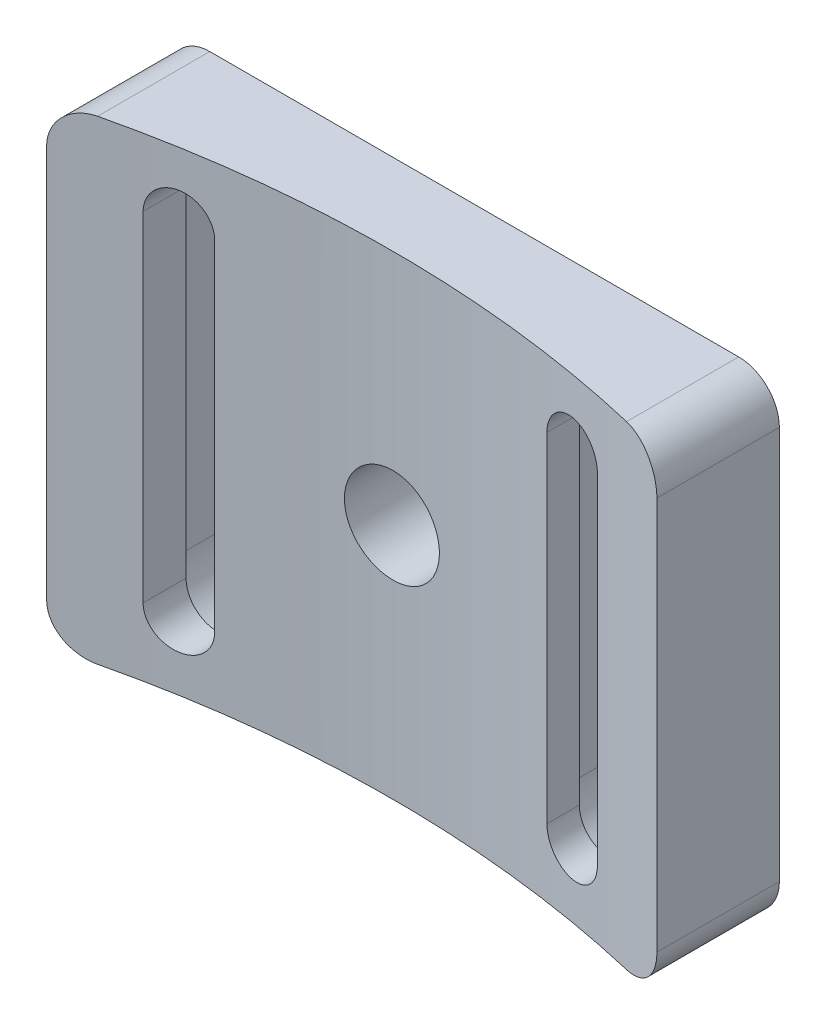
from build123d import *

# Parameters (mm, degrees)
BOSS_EXTRUDE1_DEPTH   = 35
FILLET1_R             = 3
M8X1_0_TAPPED_HOLE1_D = 7
CUT_EXTRUDE1_DEPTH    = 43.577310513
CUT_EXTRUDE2_DEPTH    = 4.5


with BuildPart() as part:
    # Sketch1 → Boss-Extrude1 (new body)
    with BuildSketch(Plane(origin=(0, 0, 0), x_dir=(1, 0, 0), z_dir=(0, 1, 0))):
        with BuildLine():
            Line((-22.5, 81.967981554), (-22.5, 91))
            Line((-22.5, 91), (22.5, 91))
            Line((22.5, 91), (22.5, 81.967981554))
            ThreePointArc((22.5, 81.967981554), (0, 85), (-22.5, 81.967981554))
        make_face()
    extrude(amount=BOSS_EXTRUDE1_DEPTH)

    # Fillet1
    fillet1_edges = [part.edges().sort_by_distance(p)[0] for p in [
        (22.5, 35, -86.483990777),
        (22.5, 0, -86.483990777),
        (-22.5, 0, -86.483990777),
        (-22.5, 35, -86.483990777),
    ]]
    fillet(fillet1_edges, radius=FILLET1_R)

    # M8x1.0 Tapped Hole1 (through all)
    with Locations(Plane(origin=(0, 0, -91), x_dir=(-1, 0, 0), z_dir=(0, 0, -1))):
        with Locations((0, 17.5)):
            Hole(M8X1_0_TAPPED_HOLE1_D / 2)

    # Sketch4 → Cut-Extrude1 (cut, through all)
    with BuildSketch(Plane(origin=(0, 0, -91), x_dir=(-1, 0, 0), z_dir=(0, 0, -1))):
        with BuildLine():
            Line((-12.25, 30), (-12.25, 5))
            ThreePointArc((-12.25, 5), (-14.5, 2.75), (-16.75, 5))
            Line((-16.75, 5), (-16.75, 30))
            ThreePointArc((-16.75, 30), (-14.5, 32.25), (-12.25, 30))
        make_face()
        with BuildLine():
            Line((16.75, 30), (16.75, 5))
            ThreePointArc((16.75, 5), (14.5, 2.75), (12.25, 5))
            Line((12.25, 5), (12.25, 30))
            ThreePointArc((12.25, 30), (14.5, 32.25), (16.75, 30))
        make_face()
    extrude(amount=-CUT_EXTRUDE1_DEPTH, mode=Mode.SUBTRACT)

    # Sketch5 → Cut-Extrude2 (cut)
    with BuildSketch(Plane(origin=(0, 0, -91), x_dir=(-1, 0, 0), z_dir=(0, 0, -1))):
        with BuildLine():
            Line((-10.5, 30), (-10.5, 5))
            ThreePointArc((-10.5, 5), (-14.5, 1), (-18.5, 5))
            Line((-18.5, 5), (-18.5, 30))
            ThreePointArc((-18.5, 30), (-14.5, 34), (-10.5, 30))
        make_face()
        with BuildLine():
            Line((18.5, 30), (18.5, 5))
            ThreePointArc((18.5, 5), (14.5, 1), (10.5, 5))
            Line((10.5, 5), (10.5, 30))
            ThreePointArc((10.5, 30), (14.5, 34), (18.5, 30))
        make_face()
    extrude(amount=-CUT_EXTRUDE2_DEPTH, mode=Mode.SUBTRACT)


solid = part.part
